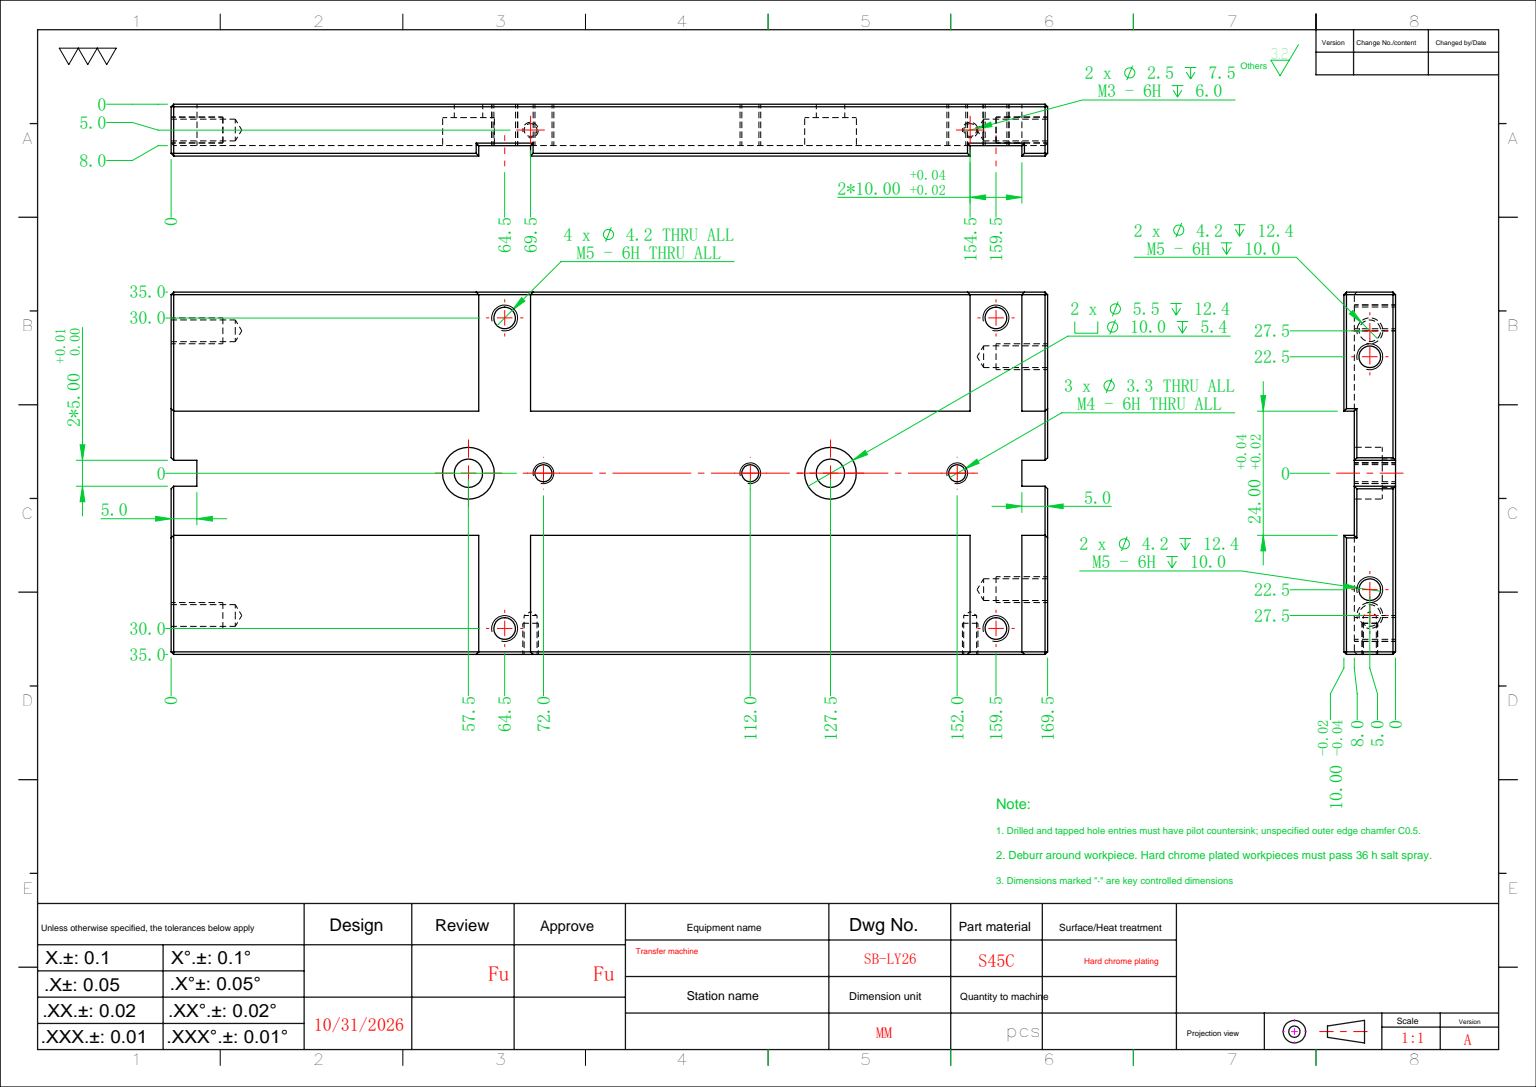
from build123d import *

# Parameters (mm, degrees)
SKETCH_1_W                     = 70
SKETCH_1_H                     = 169.5
EXTRUDE_1_DEPTH                = 10
SKETCH_2_W                     = 24
SKETCH_2_H                     = 2
CUT_EXTRUDE_1_DEPTH            = 174.364500403
SKETCH_3_W                     = 70
SKETCH_3_H                     = 10
CUT_EXTRUDE_2_DEPTH            = 2
SKETCH_4_W                     = 70
SKETCH_4_H                     = 10
CUT_EXTRUDE_3_DEPTH            = 2
HOLE_WIZARD_M5_1_D             = 4.2
HOLE_WIZARD_M4_1_D             = 3.3
HOLE_WIZARD_M5_2_D             = 4.2
HOLE_WIZARD_M5_2_DEPTH         = 12.4
HOLE_WIZARD_M5_2_TIP           = 1.2618073
SKETCH_11_W                    = 5
SKETCH_11_H                    = 8
CUT_EXTRUDE_4_DEPTH            = 5
HOLE_WIZARD_M5_3_D             = 4.2
HOLE_WIZARD_M5_3_DEPTH         = 12.4
HOLE_WIZARD_M5_3_TIP           = 1.2618073
SKETCH_14_W                    = 5
SKETCH_14_H                    = 8
CUT_EXTRUDE_5_DEPTH            = 5
HOLE_WIZARD_M5_1_2_D           = 5.5
HOLE_WIZARD_M5_1_2_DEPTH       = 12.4
HOLE_WIZARD_M5_1_2_CBORE_D     = 10
HOLE_WIZARD_M5_1_2_CBORE_DEPTH = 5.4
HOLE_WIZARD_M5_1_2_TIP         = 1.652366702
HOLE_WIZARD_M3_1_D             = 2.5
HOLE_WIZARD_M3_1_DEPTH         = 7.5
HOLE_WIZARD_M3_1_TIP           = 0.751075774
CHAMFER_1_SIZE                 = 0.5


with BuildPart() as part:
    # 草图1 → 凸台-拉伸1 (new body)
    with BuildSketch(Plane.XY):
        Rectangle(SKETCH_1_W, SKETCH_1_H)
    extrude(amount=EXTRUDE_1_DEPTH)

    # 草图2 → 切除-拉伸1 (cut, through all)
    with BuildSketch(Plane.XZ.offset(84.75)):
        with Locations((0, 1)):
            Rectangle(SKETCH_2_W, SKETCH_2_H)
    extrude(amount=-CUT_EXTRUDE_1_DEPTH, mode=Mode.SUBTRACT)

    # 草图3 → 切除-拉伸2 (cut)
    with BuildSketch(Plane(origin=(0, 0, 0), x_dir=(-1, 0, 0), z_dir=(0, 0, -1))):
        with Locations((0, 74.75)):
            Rectangle(SKETCH_3_W, SKETCH_3_H)
    extrude(amount=-CUT_EXTRUDE_2_DEPTH, mode=Mode.SUBTRACT)

    # 草图4 → 切除-拉伸3 (cut)
    with BuildSketch(Plane(origin=(0, 0, 0), x_dir=(-1, 0, 0), z_dir=(0, 0, -1))):
        with Locations((0, -20.25)):
            Rectangle(SKETCH_4_W, SKETCH_4_H)
    extrude(amount=-CUT_EXTRUDE_3_DEPTH, mode=Mode.SUBTRACT)

    # Hole Wizard M5 _1 (through all)
    with Locations(Plane(origin=(0, 0, 0), x_dir=(-1, 0, 0), z_dir=(0, 0, -1))):
        with Locations((-30, -20.25), (30, -20.25), (-30, 74.75), (30, 74.75)):
            Hole(HOLE_WIZARD_M5_1_D / 2)

    # M4 螺纹孔1 (through all)
    with Locations(Plane(origin=(0, 0, 2), x_dir=(-1, 0, 0), z_dir=(0, 0, -1))):
        with Locations((0, -12.75), (0, 27.25), (0, 67.25)):
            Hole(HOLE_WIZARD_M4_1_D / 2)

    # M5 螺纹孔2
    with Locations(Plane(origin=(0, -84.75, 0), x_dir=(-1, 0, 0), z_dir=(0, -1, 0))):
        with Locations((-27.5, -5), (27.5, -5)):
            Hole(HOLE_WIZARD_M5_2_D / 2, depth=HOLE_WIZARD_M5_2_DEPTH)
            with Locations((0, 0, -(HOLE_WIZARD_M5_2_DEPTH + HOLE_WIZARD_M5_2_TIP / 2))):  # 118° drill point
                Cone(0, HOLE_WIZARD_M5_2_D / 2, HOLE_WIZARD_M5_2_TIP, mode=Mode.SUBTRACT)

    # 草图11 → 切除-拉伸4 (cut)
    with BuildSketch(Plane.XZ.offset(84.75)):
        with Locations((0, 6)):
            Rectangle(SKETCH_11_W, SKETCH_11_H)
    extrude(amount=-CUT_EXTRUDE_4_DEPTH, mode=Mode.SUBTRACT)

    # M5 螺纹孔3
    with Locations(Plane(origin=(0, 84.75, 0), x_dir=(1, 0, 0), z_dir=(0, 1, 0))):
        with Locations((22.5, -5), (-22.5, -5)):
            Hole(HOLE_WIZARD_M5_3_D / 2, depth=HOLE_WIZARD_M5_3_DEPTH)
            with Locations((0, 0, -(HOLE_WIZARD_M5_3_DEPTH + HOLE_WIZARD_M5_3_TIP / 2))):  # 118° drill point
                Cone(0, HOLE_WIZARD_M5_3_D / 2, HOLE_WIZARD_M5_3_TIP, mode=Mode.SUBTRACT)

    # 草图14 → 切除-拉伸5 (cut)
    with BuildSketch(Plane(origin=(0, 84.75, 0), x_dir=(1, 0, 0), z_dir=(0, 1, 0))):
        with Locations((0, -6)):
            Rectangle(SKETCH_14_W, SKETCH_14_H)
    extrude(amount=-CUT_EXTRUDE_5_DEPTH, mode=Mode.SUBTRACT)

    # Hole Wizard M5 _1 2
    with Locations(Plane(origin=(0, 0, 2), x_dir=(-1, 0, 0), z_dir=(0, 0, -1))):
        with Locations((0, -27.250039646), (0, 42.749960354)):
            CounterBoreHole(HOLE_WIZARD_M5_1_2_D / 2, HOLE_WIZARD_M5_1_2_CBORE_D / 2, HOLE_WIZARD_M5_1_2_CBORE_DEPTH, depth=HOLE_WIZARD_M5_1_2_DEPTH)
            with Locations((0, 0, -(HOLE_WIZARD_M5_1_2_DEPTH + HOLE_WIZARD_M5_1_2_TIP / 2))):  # 118° drill point
                Cone(0, HOLE_WIZARD_M5_1_2_D / 2, HOLE_WIZARD_M5_1_2_TIP, mode=Mode.SUBTRACT)

    # M3 螺纹孔1
    with Locations(Plane.ZY.offset(35)):
        with Locations((5, -15.25), (5, 69.75)):
            Hole(HOLE_WIZARD_M3_1_D / 2, depth=HOLE_WIZARD_M3_1_DEPTH)
            with Locations((0, 0, -(HOLE_WIZARD_M3_1_DEPTH + HOLE_WIZARD_M3_1_TIP / 2))):  # 118° drill point
                Cone(0, HOLE_WIZARD_M3_1_D / 2, HOLE_WIZARD_M3_1_TIP, mode=Mode.SUBTRACT)

    # 倒角1
    chamfer_1_edges = [part.edges().sort_by_distance(p)[0] for p in [
        (-35, 0, 10),
        (23.5, -84.75, 0),
        (-7.25, -84.75, 2),
        (18.75, -84.75, 10),
        (-23.5, 84.75, 0),
        (-2.5, -84.75, 6),
        (2.5, -84.75, 6),
        (-18.75, -84.75, 10),
        (-7.25, 84.75, 2),
        (-18.75, 84.75, 10),
        (-2.5, 84.75, 6),
        (2.5, 84.75, 6),
        (12, 84.75, 1),
        (-12, 84.75, 1),
        (7.25, 84.75, 2),
        (12, -84.75, 1),
        (7.25, -84.75, 2),
        (-12, -84.75, 1),
        (-35, 27.25, 0),
        (35, 82.25, 0),
        (35, 79.75, 1),
        (-35, 69.75, 1),
        (35, 74.75, 2),
        (35, 69.75, 1),
        (-35, 74.75, 2),
        (-35, 79.75, 1),
        (35, 0, 10),
        (-23.5, -84.75, 0),
        (-35, 82.25, 0),
        (23.5, 84.75, 0),
        (35, -55, 0),
        (-35, -55, 0),
        (35, 27.25, 0),
        (35, -15.25, 1),
        (-35, -25.25, 1),
        (35, -20.25, 2),
        (35, -25.25, 1),
        (-35, -20.25, 2),
        (-35, -15.25, 1),
        (35, -84.75, 5),
        (-35, -84.75, 5),
        (-35, 84.75, 5),
        (35, 84.75, 5),
        (18.75, 84.75, 10),
    ]]
    chamfer(chamfer_1_edges, length=CHAMFER_1_SIZE)


solid = part.part
